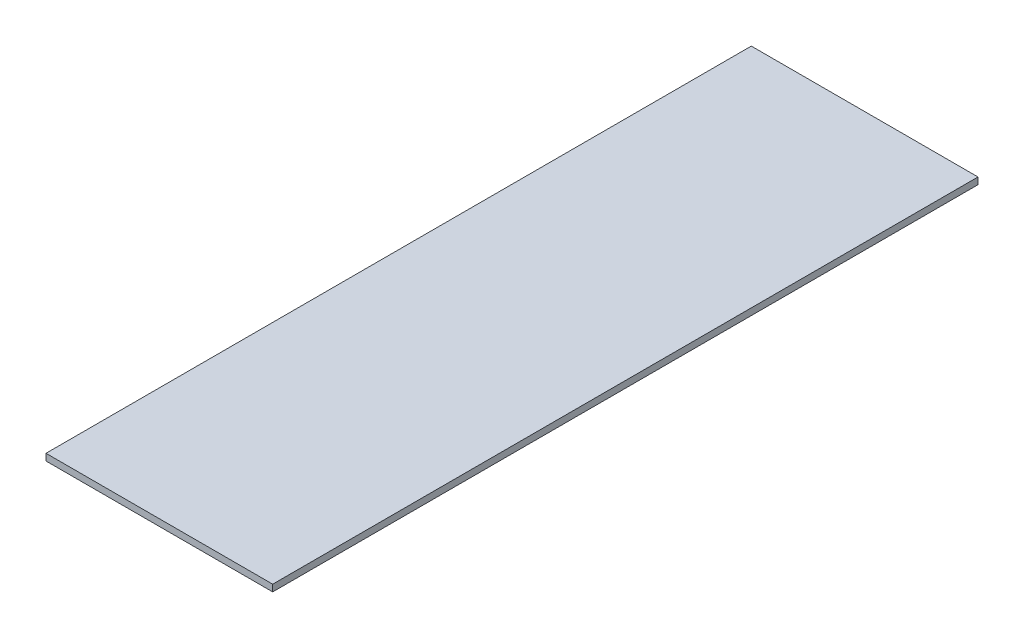
SolidWorks part; units mm, degrees
material "Q235"
ref_plane "Front Plane" through (0, 0, 0) normal (0, 0, 1) x (1, 0, 0)
ref_plane "Top Plane" through (0, 0, 0) normal (0, 1, 0) x (1, 0, 0)
ref_plane "Right Plane" through (0, 0, 0) normal (1, 0, 0) x (0, 0, -1)
sketch "Sketch1" plane through (0, 0, 0) normal (0, 1, 0) x (1, 0, 0)
  line L1 (-67.5, 210) -> (67.5, 210)
  line L2 (-67.5, 210) -> (-67.5, -210)
  line L3 (-67.5, -210) -> (67.5, -210)
  line L4 (67.5, 210) -> (67.5, -210)
  line L5 (-67.5, 210) -> (67.5, -210) construction
  line L6 (-67.5, -210) -> (67.5, 210) construction
  point P0 (0, 0)
  dimension "D1" = 420
  dimension "D2" = 135
extrude "Boss-Extrude1" add sketch "Sketch1" along normal blind 4
sketch "Sketch2" plane through (0, 4, 0) normal (0, 1, 0) x (1, 0, 0)
  line L0 (0, 0) -> (-67.5, 0) construction
  line L1 (-67.5, 210) -> (-17.5, 210)
  line L2 (-67.5, 210) -> (-67.5, 160)
  line L3 (-67.5, 160) -> (-17.5, 160)
  line L4 (-17.5, 210) -> (-17.5, 160)
  line L5 (-67.5, 210) -> (-67.5, -210) construction
  line L6 (-17.5, -210) -> (-17.5, -160)
  line L7 (-67.5, -160) -> (-17.5, -160)
  line L8 (-67.5, -210) -> (-67.5, -160)
  line L9 (-67.5, -210) -> (-17.5, -210)
  dimension "D1" = 50
  dimension "D2" = 50
extrude "Cut-Extrude1" [suppressed] cut sketch "Sketch2" against normal blind 10
